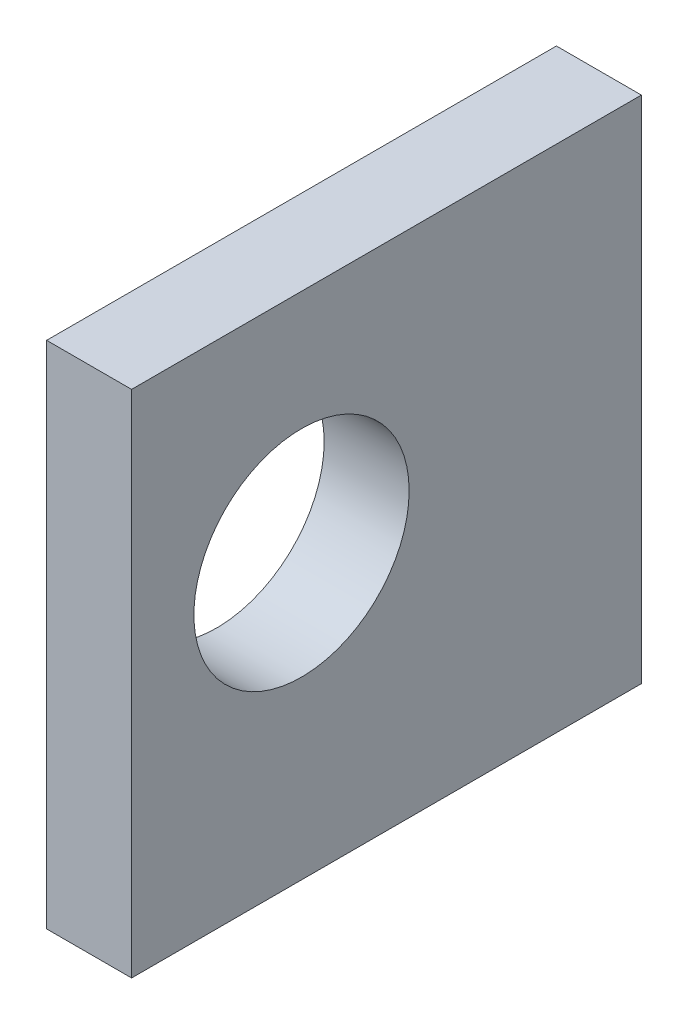
from build123d import *

# Parameters (mm, degrees)
SKETCH1_W           = 90
SKETCH1_H           = 90
BOSS_EXTRUDE1_DEPTH = 7.5
SKETCH2_R           = 19
CUT_EXTRUDE1_DEPTH  = 15


with BuildPart() as part:
    # Sketch1 → Boss-Extrude1 (new, symmetric)
    with BuildSketch(Plane(origin=(0, 0, 0), x_dir=(0, 0, -1), z_dir=(1, 0, 0))):
        Rectangle(SKETCH1_W, SKETCH1_H)
    extrude(amount=BOSS_EXTRUDE1_DEPTH, both=True)

    # Sketch2 → Cut-Extrude1 (cut)
    with BuildSketch(Plane(origin=(7.5, 0, 0), x_dir=(0, 0, -1), z_dir=(1, 0, 0))):
        with Locations((-15, 5)):
            Circle(SKETCH2_R)
    extrude(amount=-CUT_EXTRUDE1_DEPTH, mode=Mode.SUBTRACT)


solid = part.part
